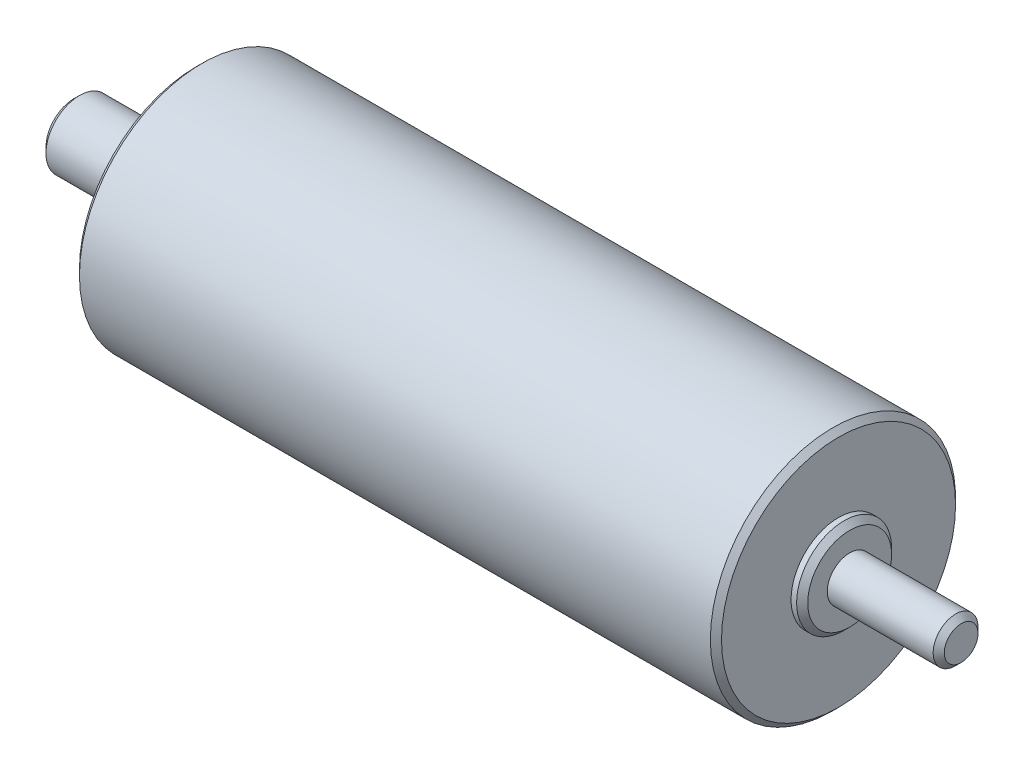
SolidWorks part; units mm, degrees
ref_plane "Front Plane" through (0, 0, 0) normal (0, 0, 1) x (1, 0, 0)
ref_plane "Top Plane" through (0, 0, 0) normal (0, 1, 0) x (1, 0, 0)
ref_plane "Right Plane" through (0, 0, 0) normal (1, 0, 0) x (0, 0, -1)
sketch "Sketch1" plane through (0, 0, 0) normal (0, 0, 1) x (1, 0, 0)
  line L0 (0, 0) -> (90.7726, 0) construction
  line L1 (0, 0) -> (0, 3)
  line L2 (0, 3) -> (10, 3)
  line L3 (10, 3) -> (10, 5.25)
  line L4 (10, 5.25) -> (11, 5.25)
  line L5 (11, 5.25) -> (11, 11)
  line L6 (11, 11) -> (68.6, 11)
  line L7 (68.6, 11) -> (68.6, 4.2618)
  line L8 (68.6, 4.2618) -> (69.6, 4.2618)
  line L9 (69.6, 4.2618) -> (69.6, 2.0118)
  line L10 (69.6, 2.0118) -> (79.6, 2.0118)
  line L11 (79.6, 2.0118) -> (79.6, 0)
  line L12 (0, 0) -> (79.6, 0)
  dimension "D1" = 79.6
  dimension "D2" = 59.6
  dimension "D3" = 57.6
  dimension "D4" = 11
  dimension "D5" = 3
  dimension "D6" = 5.25
revolve "Revolve1" add sketch "Sketch1" angle 360 about L0
chamfer "Chamfer1" distance 0.5 angle 45 6 edges at (0, 0, 3) (10, 0, 5.25) (11, 0, 11) (68.6, 0, 11) (69.6, 0, 4.2618) (79.6, 0, 2.0118)
